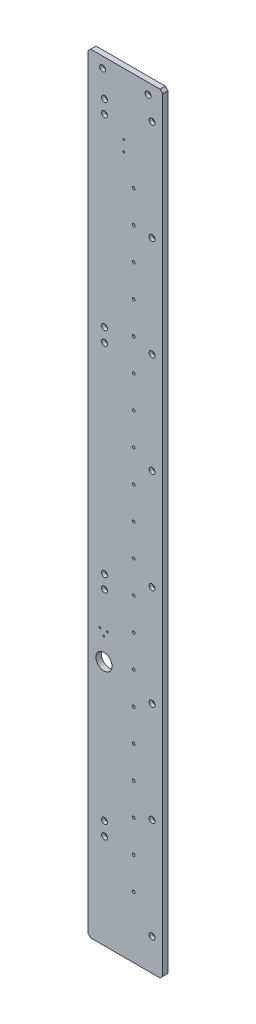
SolidWorks part; units mm, degrees
material "6061-T6"
ref_plane "前视基准面" through (0, 0, 0) normal (0, 0, 1) x (1, 0, 0)
ref_plane "上视基准面" through (0, 0, 0) normal (0, 1, 0) x (1, 0, 0)
ref_plane "右视基准面" through (0, 0, 0) normal (1, 0, 0) x (0, 0, -1)
sketch "草图1" plane through (0, 0, 0) normal (0, 0, 1) x (1, 0, 0)
  line L1 (0, 0) -> (140, 0)
  line L2 (0, 0) -> (0, -1440)
  line L3 (0, -1440) -> (140, -1440)
  line L4 (140, 0) -> (140, -1440)
  dimension "D1" = 1440
  dimension "D2" = 140
extrude "凸台-拉伸1" add sketch "草图1" along normal blind 10
hole_wizard "M6 螺纹孔1" positions "草图2" profile "草图3" tap size "M6" standard "ISO" end condition through all
sketch "草图2" plane through (0, 0, 10) normal (0, 0, 1) x (1, 0, 0)
  line L0 (140, 0) -> (0, 0) construction
  line L1 (140, -1440) -> (140, 0) construction
  point P0 (85.75, -185)
  point P14 (85.75, -245)
  point P15 (85.75, -305)
  point P16 (85.75, -365)
  point P17 (85.75, -425)
  point P18 (85.75, -485)
  point P19 (85.75, -545)
  point P20 (85.75, -605)
  point P21 (85.75, -665)
  point P22 (85.75, -725)
  point P23 (85.75, -785)
  point P24 (85.75, -845)
  point P25 (85.75, -905)
  point P26 (85.75, -965)
  point P27 (85.75, -1025)
  point P28 (85.75, -1085)
  point P29 (85.75, -1145)
  point P30 (85.75, -1205)
  point P31 (85.75, -1265)
  point P32 (85.75, -1325)
  dimension "D1" = 185
  dimension "D2" = 54.25
  dimension "D4" = 60
  dimension "D3" = 20
sketch "草图3" plane through (85.75, -185, 10) normal (1, 0, 0) x (0, -1, 0)
  line L0 (0, 0) -> (0, 10)
  line L1 (0, 10) -> (2.5, 10)
  line L2 (2.5, 10) -> (2.5, 0)
  line L5 (2.5, 0) -> (0, 0)
  line L11 (0, -6.35) -> (0, 107.95) construction
  dimension "通孔螺纹孔钻头直径" = 5
  dimension "通孔螺纹孔钻头深度" = 10
cosmetic thread "孔螺蚊线1"
cosmetic thread "孔螺蚊线2"
cosmetic thread "孔螺蚊线3"
cosmetic thread "孔螺蚊线4"
cosmetic thread "孔螺蚊线5"
cosmetic thread "孔螺蚊线6"
cosmetic thread "孔螺蚊线7"
cosmetic thread "孔螺蚊线8"
cosmetic thread "孔螺蚊线9"
cosmetic thread "孔螺蚊线10"
cosmetic thread "孔螺蚊线11"
cosmetic thread "孔螺蚊线12"
cosmetic thread "孔螺蚊线13"
cosmetic thread "孔螺蚊线14"
cosmetic thread "孔螺蚊线15"
cosmetic thread "孔螺蚊线16"
cosmetic thread "孔螺蚊线17"
cosmetic thread "孔螺蚊线18"
cosmetic thread "孔螺蚊线19"
cosmetic thread "孔螺蚊线20"
hole_wizard "M6 六角凹头螺钉的柱形沉头孔1" positions "草图4" profile "草图5" counterbore size "M6" standard "ISO"
sketch "草图4" plane through (0, 0, 10) normal (0, 0, 1) x (1, 0, 0)
  line L0 (31, -1262.5) -> (31, -1237.5) construction
  line L2 (0, 0) -> (0, -1440) construction
  line L3 (0, -1440) -> (140, -1440) construction
  line L4 (31, -437.5) -> (31, -92.5) construction
  line L6 (31, -92.5) -> (31, -67.5) construction
  point P0 (31, -1262.5)
  point P2 (31, -1237.5)
  point P20 (31, -862.5)
  point P21 (31, -837.5)
  point P22 (31, -462.5)
  point P23 (31, -437.5)
  point P24 (31, -92.5)
  point P25 (31, -67.5)
  dimension "D1" = 31
  dimension "D2" = 25
  dimension "D3" = 177.5
  dimension "D5" = 345
  dimension "D4" = 25
sketch "草图5" plane through (31, -1262.5, 10) normal (1, 0, 0) x (0, -1, 0)
  line L0 (0, 0) -> (0, 18.9828)
  line L1 (0, 18.9828) -> (3.3, 17)
  line L2 (3.3, 17) -> (3.3, 6.4)
  line L3 (3.3, 6.4) -> (5.5, 6.4)
  line L4 (5.5, 6.4) -> (5.5, 0)
  line L5 (5.5, 0) -> (0, 0)
  line L10 (0, 18.9828) -> (-3.3, 17) construction
  line L11 (0, -6.35) -> (0, 107.95) construction
  dimension "孔直径" = 6.6
  dimension "孔深度" = 17
  dimension "柱形沉头孔直径" = 11
  dimension "柱形沉头孔深度" = 6.4
  dimension "导头角度" = 118
hole_wizard "M4 螺纹孔1" positions "草图7" profile "草图8" tap size "M4" standard "ISO" end condition through all
sketch "草图7" plane through (0, 0, 10) normal (0, 0, 1) x (1, 0, 0)
  line L0 (22.5, -928.5) -> (29.5, -938.5) construction
  line L1 (29.5, -938.5) -> (36.5, -928.5) construction
  line L2 (36.5, -928.5) -> (22.5, -928.5) construction
  line L4 (29.5, -938.5) -> (29.5, -928.5) construction
  line L6 (0, 0) -> (0, -1440) construction
  point P0 (22.5, -928.5)
  point P2 (36.5, -928.5)
  point P4 (29.5, -938.5)
  dimension "D1" = 14
  dimension "D2" = 10
  dimension "D3" = 29.5
sketch "草图8" plane through (22.5, -928.5, 10) normal (1, 0, 0) x (0, -1, 0)
  line L0 (0, 0) -> (0, 10)
  line L1 (0, 10) -> (1.65, 10)
  line L2 (1.65, 10) -> (1.65, 0)
  line L5 (1.65, 0) -> (0, 0)
  line L11 (0, -6.35) -> (0, 107.95) construction
  dimension "通孔螺纹孔钻头直径" = 3.3
  dimension "通孔螺纹孔钻头深度" = 10
cosmetic thread "孔螺蚊线21"
cosmetic thread "孔螺蚊线22"
cosmetic thread "孔螺蚊线23"
sketch "草图9" plane through (0, 0, 10) normal (0, 0, 1) x (1, 0, 0)
  line L0 (0, 0) -> (0, -1440) construction
  line L1 (0, -1440) -> (140, -1440) construction
  circle A0 centre (30, -980) radius 15
  dimension "D3" = 30
  dimension "D1" = 30
  dimension "D2" = 460
extrude "切除-拉伸2" cut sketch "草图9" against normal blind 10
chamfer "倒角1" distance 5 angle 45 4 edges at (140, 0, 5) (0, 0, 5) (0, -1440, 5) (140, -1440, 5)
hole_wizard "M6 六角凹头螺钉的柱形沉头孔2" positions "草图10" profile "草图11" counterbore size "M6" standard "ISO"
sketch "草图10" plane through (0, 0, 10) normal (0, 0, 1) x (1, 0, 0)
  line L0 (140, -1435) -> (140, -5) construction
  line L2 (120, -1380) -> (120, -60) construction
  line L4 (120, -720) -> (140, -720) construction
  line L7 (5, -1440) -> (135, -1440) construction
  line L9 (27.5, -20) -> (112.5, -20) construction
  line L11 (70, -20) -> (70, 0) construction
  line L12 (135, 0) -> (5, 0) construction
  point P0 (120, -1380)
  point P14 (120, -1191.4286)
  point P15 (120, -1002.8571)
  point P16 (120, -814.2857)
  point P17 (120, -625.7143)
  point P18 (120, -437.1429)
  point P19 (120, -248.5714)
  point P20 (120, -60)
  point P35 (27.5, -20)
  point P37 (112.5, -20)
  dimension "D1" = 20
  dimension "D2" = 60
  dimension "D4" = 20
  dimension "D5" = 85
  dimension "D3" = 8
sketch "草图11" plane through (120, -1380, 10) normal (1, 0, 0) x (0, -1, 0)
  line L0 (0, 0) -> (0, 18.9828)
  line L1 (0, 18.9828) -> (3.3, 17)
  line L2 (3.3, 17) -> (3.3, 6.4)
  line L3 (3.3, 6.4) -> (5.5, 6.4)
  line L4 (5.5, 6.4) -> (5.5, 0)
  line L5 (5.5, 0) -> (0, 0)
  line L10 (0, 18.9828) -> (-3.3, 17) construction
  line L11 (0, -6.35) -> (0, 107.95) construction
  dimension "孔直径" = 6.6
  dimension "孔深度" = 17
  dimension "柱形沉头孔直径" = 11
  dimension "柱形沉头孔深度" = 6.4
  dimension "导头角度" = 118
hole_wizard "M4 螺纹孔2" positions "草图12" profile "草图13" tap size "M4" standard "ISO"
sketch "草图12" plane through (0, 0, 10) normal (0, 0, 1) x (1, 0, 0)
  line L0 (67, -135.5) -> (67, -115.5) construction
  line L2 (0, -5) -> (0, -1435) construction
  point P0 (67, -115.5)
  point P2 (67, -135.5)
  dimension "D1" = 67
sketch "草图13" plane through (67, -115.5, 10) normal (1, 0, 0) x (0, -1, 0)
  line L0 (0, 0) -> (0, 12.4914)
  line L1 (0, 12.4914) -> (1.65, 11.5)
  line L2 (1.65, 11.5) -> (1.65, 0)
  line L5 (1.65, 0) -> (0, 0)
  line L10 (0, 12.4914) -> (-1.65, 11.5) construction
  line L11 (0, -6.35) -> (0, 107.95) construction
  dimension "螺纹孔钻头直径" = 3.3
  dimension "螺纹孔钻头深度" = 11.5
  dimension "导头角度" = 118
cosmetic thread "孔螺蚊线24"
cosmetic thread "孔螺蚊线25"
